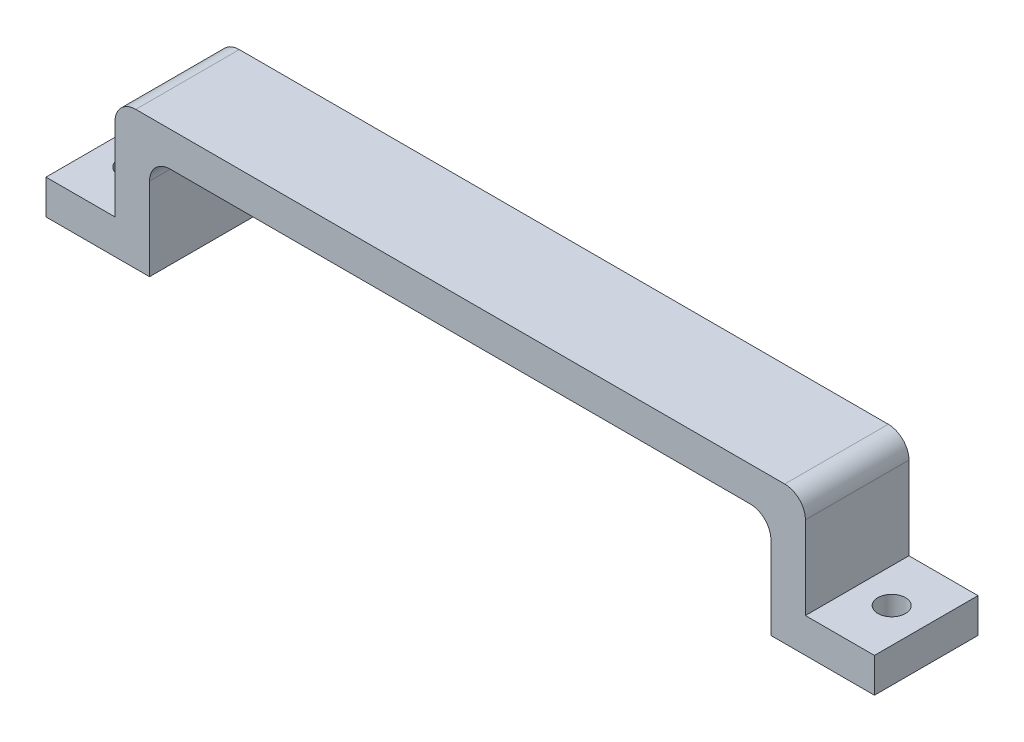
SolidWorks part; units mm, degrees
ref_plane "前视" through (0, 0, 0) normal (0, 0, 1) x (1, 0, 0)
ref_plane "上视" through (0, 0, 0) normal (0, 1, 0) x (1, 0, 0)
ref_plane "右视" through (0, 0, 0) normal (1, 0, 0) x (0, 0, -1)
sketch "草图1" plane through (0, 0, 0) normal (0, 0, 1) x (1, 0, 0)
  line L0 (0, 0) -> (15, 0)
  line L1 (15, 0) -> (15, 15)
  line L2 (15, 15) -> (105, 15)
  line L3 (105, 15) -> (105, 0)
  line L4 (105, 0) -> (120, 0)
  line L5 (120, 0) -> (120, 5)
  line L6 (120, 5) -> (110, 5)
  line L7 (110, 5) -> (110, 20)
  line L8 (0, 0) -> (0, 5)
  line L9 (0, 5) -> (10, 5)
  line L10 (10, 5) -> (10, 20)
  line L11 (10, 20) -> (110, 20)
  dimension "D1" = 120
  dimension "D2" = 15
  dimension "D3" = 15
  dimension "D4" = 10
  dimension "D5" = 10
  dimension "D6" = 15
  dimension "D7" = 20
  dimension "D8" = 5
  dimension "D9" = 5
extrude "凸台-拉伸1" add sketch "草图1" along normal blind 15
sketch "草图2" plane through (0, 5, 0) normal (0, 1, 0) x (1, 0, 0)
  line L0 (120, -7.5) -> (-6.4998, -7.5) construction
  line L1 (120, -15) -> (120, 0) construction
  line L2 (0, -15) -> (0, 0) construction
  circle A0 centre (5, -7.5) radius 2
  circle A1 centre (115, -7.5) radius 2
  dimension "D1" = 4
  dimension "D2" = 4
  dimension "D3" = 5
  dimension "D4" = 5
extrude "切除-拉伸1" cut sketch "草图2" against normal blind 15
fillet "圆角1" radius 3 4 edges at (110, 20, 7.5) (10, 20, 7.5) (105, 15, 7.5) (15, 15, 7.5)
